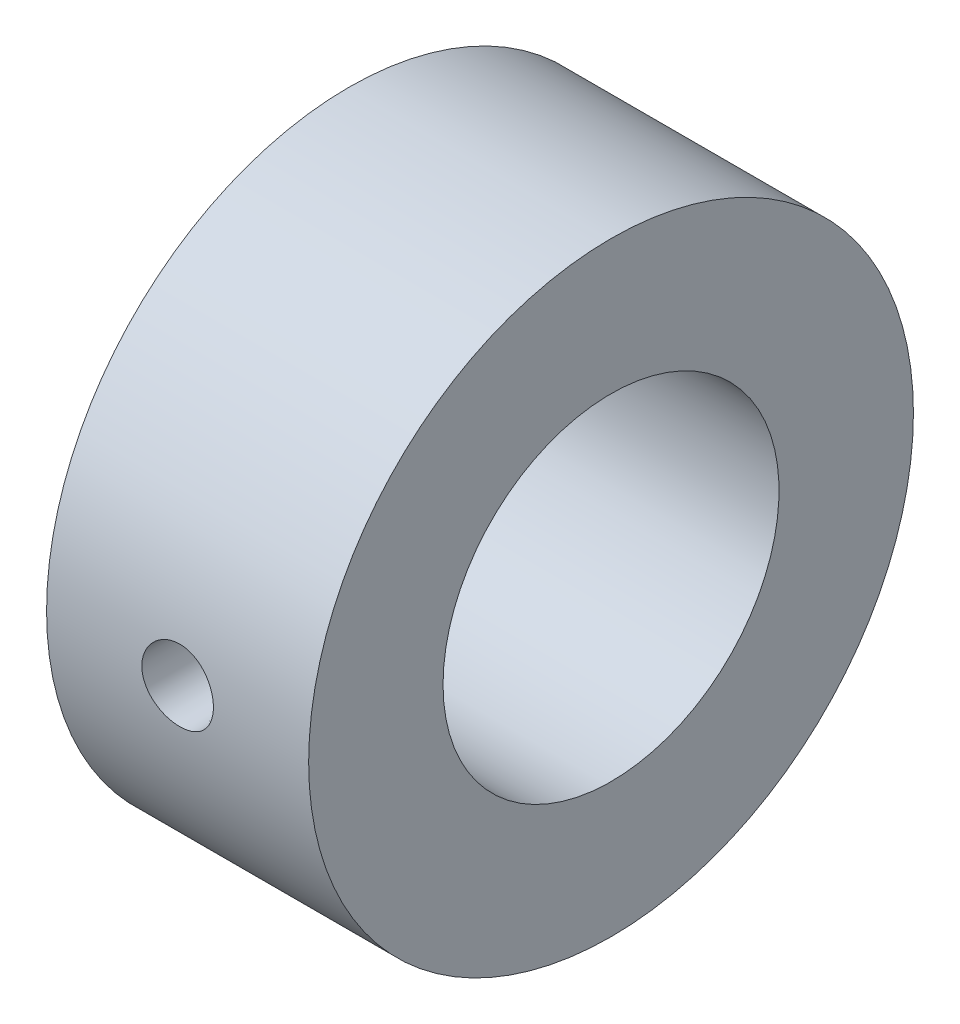
from build123d import *

# Parameters (mm, degrees)
SKETCH1_R           = 45
SKETCH1_R_2         = 25
BOSS_EXTRUDE1_DEPTH = 39


with BuildPart() as part:
    # Sketch1 → Boss-Extrude1 (new body)
    with BuildSketch(Plane.ZY.offset(-128)):
        with Locations((-102.5, 90)):
            Circle(SKETCH1_R)
        with Locations((-102.5, 90)):
            Circle(SKETCH1_R_2, mode=Mode.SUBTRACT)
    extrude(amount=-BOSS_EXTRUDE1_DEPTH)

    # Sketch2 → Cut-Revolve1 (revolve, cut)
    with BuildSketch(Plane(origin=(147.5, 0, 0), x_dir=(0, 0, -1), z_dir=(1, 0, 0)), mode=Mode.PRIVATE) as cut_revolve1_sk:
        Polygon((0, 90), (0, 95.9), (90, 95), (90, 90), align=None)
    revolve(cut_revolve1_sk.sketch.rotate(Axis((147.5, 90, -102.5), (0, 0, 1)), 269.999999962), axis=Axis((147.5, 90, -102.5), (0, 0, 1)), mode=Mode.SUBTRACT)


solid = part.part
